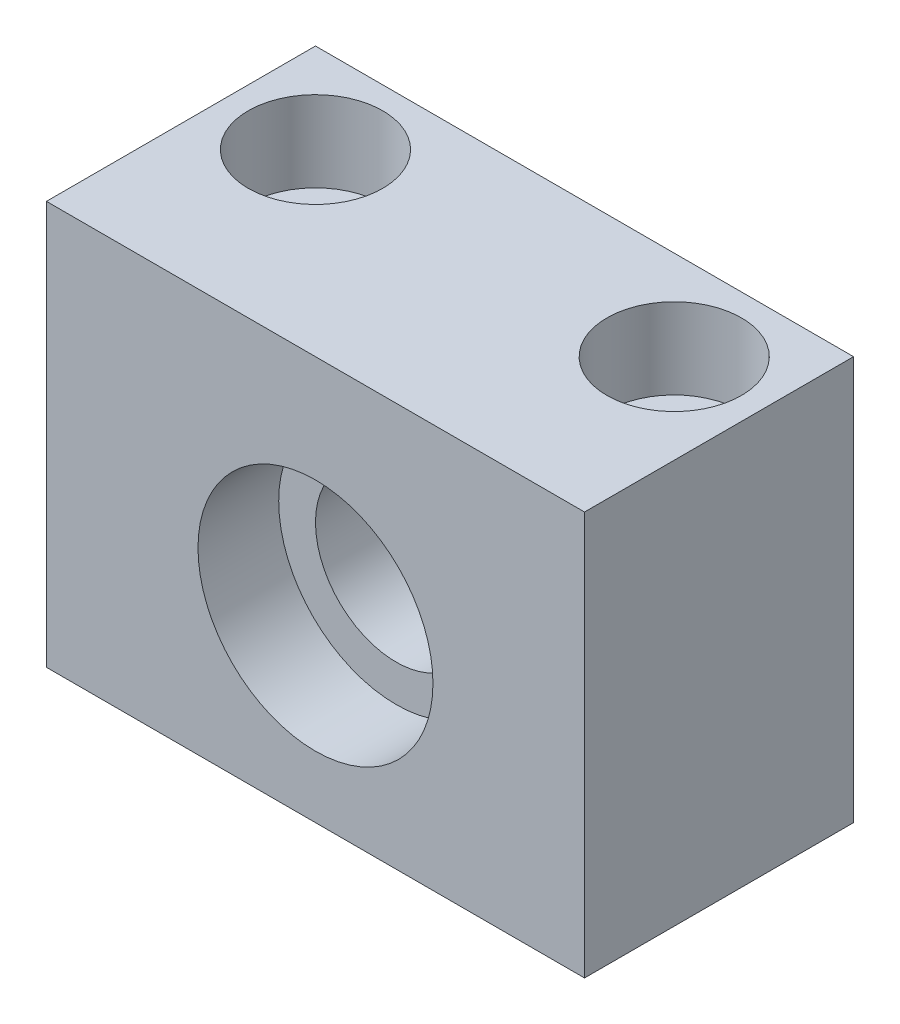
from build123d import *

# Parameters (mm, degrees)
SKETCH1_W                                            = 60
SKETCH1_H                                            = 45
SKETCH1_R                                            = 9
BOSS_EXTRUDE1_DEPTH                                  = 30
HOLE_SIZE_PER_SOCKET_HEAD_CAP_SCREW_TYPE_D           = 9
HOLE_SIZE_PER_SOCKET_HEAD_CAP_SCREW_TYPE_CBORE_D     = 15
HOLE_SIZE_PER_SOCKET_HEAD_CAP_SCREW_TYPE_CBORE_DEPTH = 9
SKETCH2_R                                            = 13.1
EXTRUDE1_DEPTH                                       = 9
EXTRUDE2_START                                       = -9
SKETCH3_R                                            = 13.1
EXTRUDE2_DEPTH                                       = 9


with BuildPart() as part:
    # Sketch1 → Boss-Extrude1 (new body)
    with BuildSketch(Plane.XY):
        with Locations((0, 2.5)):
            Rectangle(SKETCH1_W, SKETCH1_H)
        Circle(SKETCH1_R, mode=Mode.SUBTRACT)
    extrude(amount=BOSS_EXTRUDE1_DEPTH)

    # Hole size per socket head cap screw type1 (through all)
    with Locations(Plane(origin=(0, 25, 0), x_dir=(-1, 0, 0), z_dir=(0, 1, 0))):
        with Locations((20, 10), (-20, 10)):
            CounterBoreHole(HOLE_SIZE_PER_SOCKET_HEAD_CAP_SCREW_TYPE_D / 2, HOLE_SIZE_PER_SOCKET_HEAD_CAP_SCREW_TYPE_CBORE_D / 2, HOLE_SIZE_PER_SOCKET_HEAD_CAP_SCREW_TYPE_CBORE_DEPTH)

    # Sketch2 → Extrude1 (cut)
    with BuildSketch(Plane.XY.offset(30)):
        Circle(SKETCH2_R)
    extrude(amount=-EXTRUDE1_DEPTH, mode=Mode.SUBTRACT)

    # Sketch3 → Extrude2 (cut)
    with BuildSketch(Plane(origin=(0, 0, 0), x_dir=(-1, 0, 0), z_dir=(0, 0, -1)).offset(EXTRUDE2_START)):
        with Locations(Location((0, 0, 0), (0, 0, 180))):
            Circle(SKETCH3_R)
    extrude(amount=EXTRUDE2_DEPTH, mode=Mode.SUBTRACT)


solid = part.part
